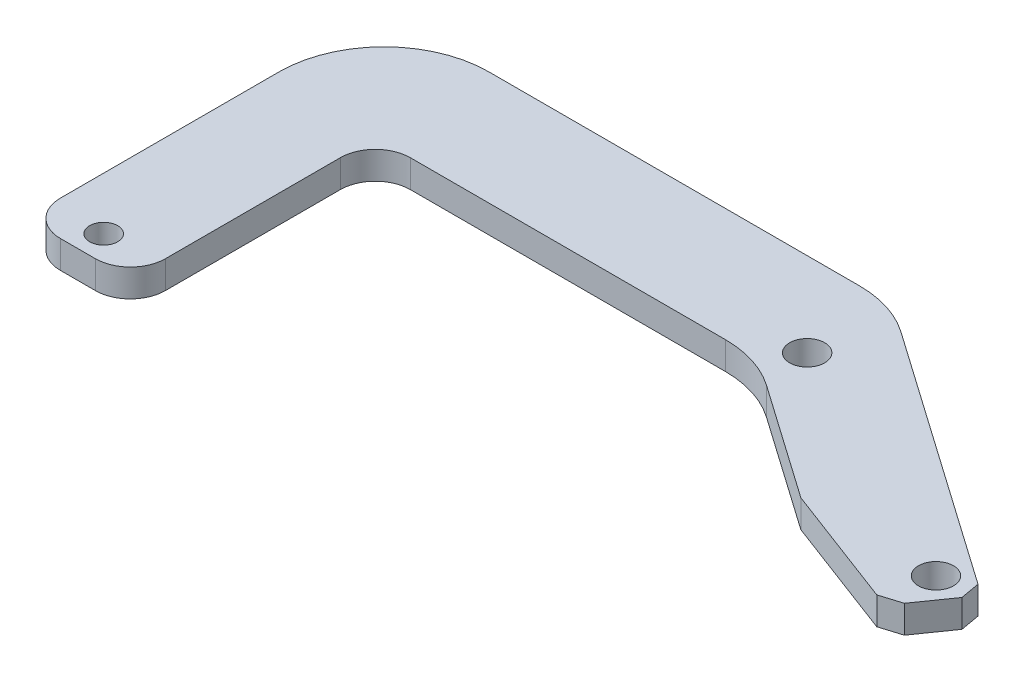
from build123d import *

# Parameters (mm, degrees)
SKETCH1_R          = 5
SKETCH1_R_2        = 4
BOSS_EXTRU_1_DEPTH = 7.9
SKETCH2_R          = 5
CUT_EXTRUDE1_DEPTH = 212.826281623
FILLET1_R          = 10


with BuildPart() as part:
    # Sketch1 → Boss.-Extru.1 (new body)
    with BuildSketch(Plane(origin=(0, 0, 0), x_dir=(1, 0, 0), z_dir=(0, 1, 0))):
        with BuildLine():
            Line((149.698750242, -34.853527415), (116.932668471, -11.910469961))
            ThreePointArc((116.932668471, -11.910469961), (108.746549365, -7.873522768), (99.72537538, -6.48503129))
            Line((99.72537538, -6.48503129), (9.72537538, -6.48503129))
            ThreePointArc((9.72537538, -6.48503129), (2.654307568, -9.413963478), (-0.27462462, -16.48503129))
            Line((-0.27462462, -16.48503129), (-0.27462462, -76.48503129))
            Line((-0.27462462, -76.48503129), (-30.27462462, -76.48503129))
            Line((-30.27462462, -76.48503129), (-30.27462462, -4.017204085))
            ThreePointArc((-30.27462462, -4.017204085), (-21.487828056, 17.195999351), (-0.27462462, 25.982795915))
            Line((-0.27462462, 25.982795915), (105.659916542, 25.982795915))
            ThreePointArc((105.659916542, 25.982795915), (114.681090527, 24.594304438), (122.867209633, 20.557357244))
            Line((122.867209633, 20.557357244), (196.395516927, -30.927717795))
            Line((196.395516927, -30.927717795), (197.377819359, -36.498631718))
            Line((197.377819359, -36.498631718), (190.606283823, -46.169386696))
            Line((190.606283823, -46.169386696), (184.570257854, -48.031947572))
            Line((184.570257854, -48.031947572), (149.698750242, -34.853527415))
        make_face()
        with Locations(Location((188.311978078, -34.853527415, 0), (0, 0, 270))):
            Circle(SKETCH1_R, mode=Mode.SUBTRACT)
        with Locations(Location((-15.27462462, -69.11920583, 0), (0, 0, 270))):
            Circle(SKETCH1_R_2, mode=Mode.SUBTRACT)
    extrude(amount=BOSS_EXTRU_1_DEPTH)

    # Sketch2 → Cut-Extrude1 (cut, through all)
    with BuildSketch(Plane.XZ):
        with Locations(Location((114.715355874, -1.93178017, 0), (0, 0, 270))):
            Circle(SKETCH2_R)
    extrude(amount=-CUT_EXTRUDE1_DEPTH, mode=Mode.SUBTRACT)

    # Fillet1
    fillet1_edges = [part.edges().sort_by_distance(p)[0] for p in [
        (-30.27462462, 3.95, 76.48503129),
        (-0.27462462, 3.95, 76.48503129),
    ]]
    fillet(fillet1_edges, radius=FILLET1_R)


solid = part.part
